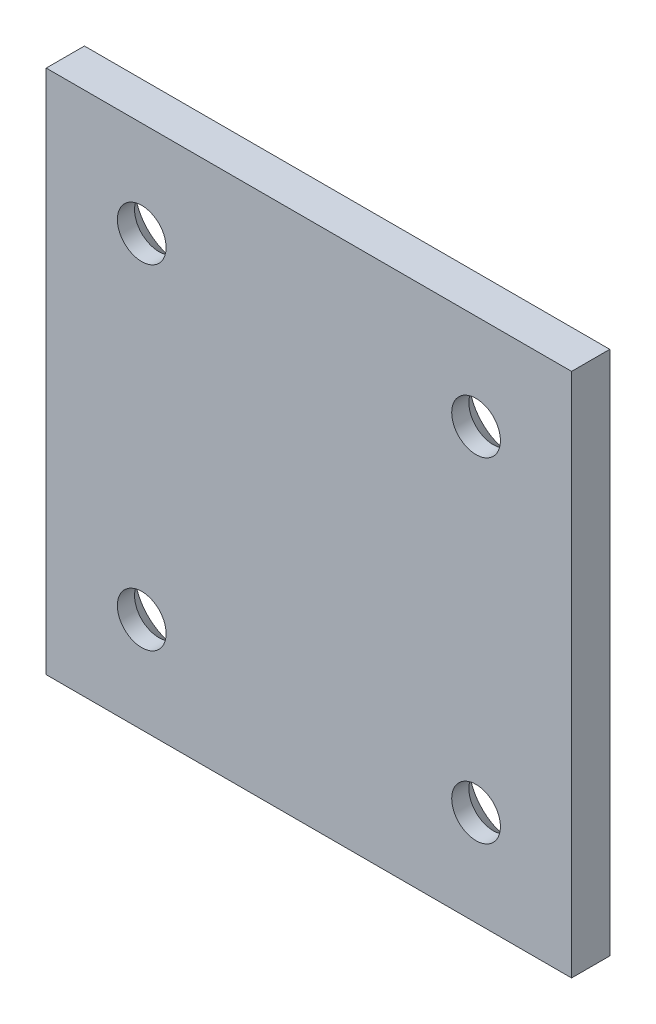
SolidWorks part; units mm, degrees
material "H62"
ref_plane "Front Plane" through (0, 0, 0) normal (0, 0, 1) x (1, 0, 0)
ref_plane "Top Plane" through (0, 0, 0) normal (0, 1, 0) x (1, 0, 0)
ref_plane "Right Plane" through (0, 0, 0) normal (1, 0, 0) x (0, 0, -1)
other "Configuration Table"
sketch "Sketch1" plane through (0, 0, 0) normal (0, 0, 1) x (1, 0, 0)
  line L1 (-27.5, -27.5) -> (27.5, -27.5)
  line L2 (-27.5, -27.5) -> (-27.5, 27.5)
  line L3 (-27.5, 27.5) -> (27.5, 27.5)
  line L4 (27.5, -27.5) -> (27.5, 27.5)
  line L5 (-27.5, -27.5) -> (27.5, 27.5) construction
  line L6 (-27.5, 27.5) -> (27.5, -27.5) construction
  line L7 (-17.5, -17.5) -> (17.5, -17.5)
  line L8 (-17.5, -17.5) -> (-17.5, 17.5)
  line L9 (-17.5, 17.5) -> (17.5, 17.5)
  line L10 (17.5, -17.5) -> (17.5, 17.5)
  line L11 (-17.5, -17.5) -> (17.5, 17.5) construction
  line L12 (-17.5, 17.5) -> (17.5, -17.5) construction
  point P0 (0, 0)
  point P6 (0, 0)
  dimension "D1" = 55
  dimension "D2" = 55
  dimension "D3" = 35
extrude "Boss-Extrude1" add sketch "Sketch1" along normal blind 4 contours L7 L10 L9 L8 | L1 L4 L3 L2 L10 L7 L8 L9
hole_wizard "Ø1.0 (5.1) Diameter Hole1" positions "Sketch2" profile "Sketch3" hole size "Ø1.0" standard "GB" end condition through all
sketch "Sketch2" plane through (0, 0, 0) normal (0, 0, -1) x (-1, 0, 0)
  point P0 (-17.5, 17.5)
  point P3 (17.5, 17.5)
  point P6 (17.5, -17.5)
  point P9 (-17.5, -17.5)
sketch "Sketch3" plane through (17.5, 17.5, 0) normal (1, 0, 0) x (0, 1, 0)
  line L0 (0, 0) -> (0, 4)
  line L1 (0, 4) -> (2.55, 4)
  line L2 (2.55, 4) -> (2.55, 0)
  line L5 (2.55, 0) -> (0, 0)
  line L11 (0, -6.35) -> (0, 107.95) construction
  dimension "通孔孔直径" = 5.1
  dimension "通孔孔深度" = 4
chamfer "Chamfer1" distance 2.2 angle 45 4 edges at (14.95, -17.5, 0) (-20.05, -17.5, 0) (-20.05, 17.5, 0) (14.95, 17.5, 0)
